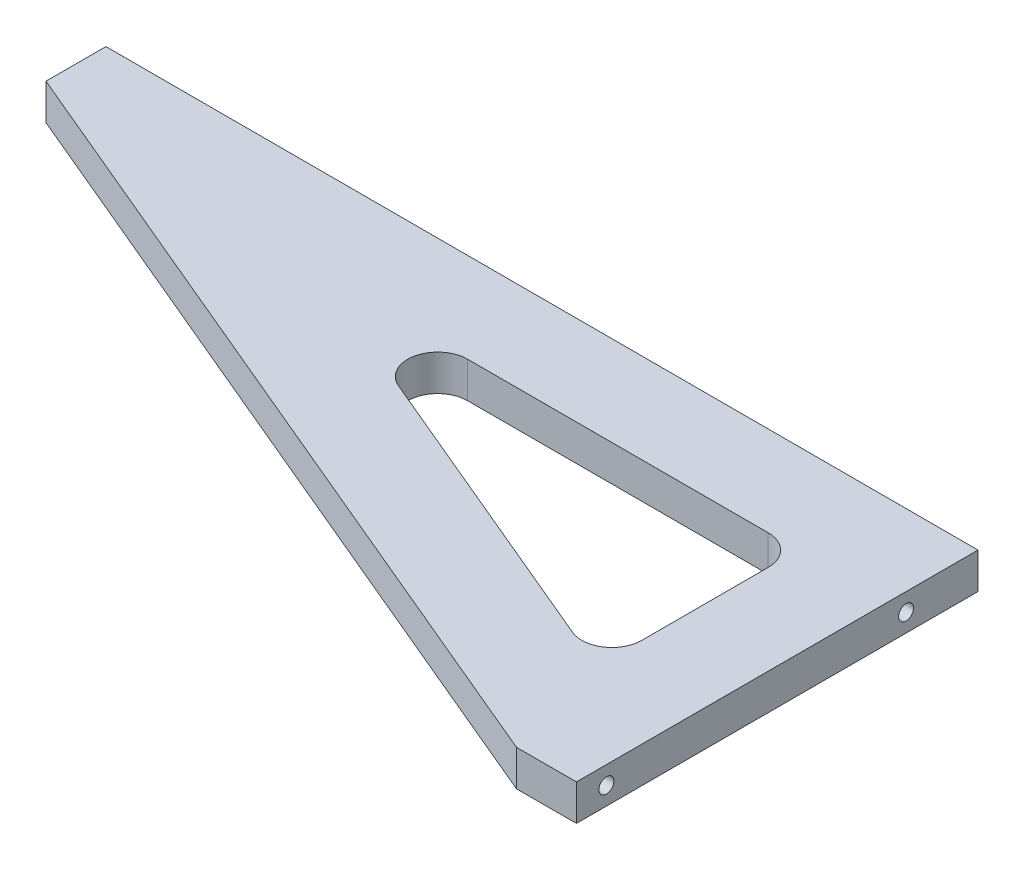
SolidWorks part; units mm, degrees
material "A6061"
ref_plane "前基準面" through (0, 0, 0) normal (0, 0, 1) x (1, 0, 0)
ref_plane "上基準面" through (0, 0, 0) normal (0, 1, 0) x (1, 0, 0)
ref_plane "右基準面" through (0, 0, 0) normal (1, 0, 0) x (0, 0, -1)
sketch "草图1" plane through (0, 0, 0) normal (0, 1, 0) x (1, 0, 0)
  line L1 (-145.5, -67) -> (145.5, -67)
  line L2 (-145.5, -67) -> (-145.5, 67)
  line L3 (-145.5, 67) -> (145.5, 67)
  line L4 (145.5, -67) -> (145.5, 67)
  line L5 (-145.5, -67) -> (145.5, 67) construction
  line L6 (-145.5, 67) -> (145.5, -67) construction
  point P0 (0, 0)
  dimension "D1" = 291
  dimension "D2" = 134
extrude "凸台-拉伸1" add sketch "草图1" along normal mid plane 12
sketch "草图2" plane through (0, 6, 0) normal (0, 1, 0) x (1, 0, 0)
  line L1 (-145.5, -67) -> (125.5, -67)
  line L2 (-145.5, -67) -> (-145.5, 47)
  line L6 (-145.5, 47) -> (125.5, -67)
  line L7 (145.5, -67) -> (145.5, 67) construction
  line L8 (145.5, 67) -> (-145.5, 67) construction
  line L9 (115.5, -15.1916) -> (115.5, 27)
  line L10 (105.5, 37) -> (5.2024, 37)
  line L11 (1.3248, 17.7824) -> (101.6225, -24.4093)
  arc A1 (5.2024, 37) -> (1.3248, 17.7824) centre (5.2024, 27) ccw
  arc A2 (115.5, 27) -> (105.5, 37) centre (105.5, 27) ccw
  arc A3 (115.5, -15.1916) -> (101.6225, -24.4093) centre (105.5, -15.1916) cw
  dimension "D3" = 30
  dimension "D6" = 10
  dimension "D1" = 20
  dimension "D2" = 20
  dimension "D4" = 30
  dimension "D5" = 30
extrude "切除-拉伸1" cut sketch "草图2" against normal through all
hole_wizard "M6 螺纹孔1" positions "草图3" profile "草图4" tap size "M6" standard "GB"
sketch "草图3" plane through (145.5, 0, 0) normal (1, 0, 0) x (0, 0, -1)
  line L0 (-67, 6) -> (-67, -6) construction
  point P0 (-57, 0)
  point P3 (43, 0)
  dimension "D2" = 10
  dimension "D3" = 100
sketch "草图4" plane through (145.5, 0, 57) normal (0, 1, 0) x (0, 0, -1)
  line L0 (0, 0) -> (0, 16.5022)
  line L1 (0, 16.5022) -> (2.5, 15)
  line L2 (2.5, 15) -> (2.5, 0)
  line L5 (2.5, 0) -> (0, 0)
  line L10 (0, 16.5022) -> (-2.5, 15) construction
  line L11 (0, -6.35) -> (0, 107.95) construction
  dimension "螺纹孔钻头直径" = 5
  dimension "螺纹孔钻头深度" = 15
  dimension "导头角度" = 118
cosmetic thread "孔螺蚊线2" parameters "D1"=12, "D2"=6
cosmetic thread "孔螺蚊线3" parameters "D1"=12, "D2"=6
hole_wizard "M6 螺纹孔2" positions "草图5" profile "草图6" tap size "M6" standard "GB"
sketch "草图5" plane through (0, 0, -67) normal (0, 0, -1) x (-1, 0, 0)
  line L0 (145.5, 6) -> (145.5, -6) construction
  point P0 (135.5, 0)
  point P5 (25.5, 0)
  point P6 (-84.5, 0)
  dimension "D2" = 10
  dimension "D3" = 110
  dimension "D1" = 3
sketch "草图6" plane through (-135.5, 0, -67) normal (1, 0, 0) x (0, 1, 0)
  line L0 (0, 0) -> (0, 16.5022)
  line L1 (0, 16.5022) -> (2.5, 15)
  line L2 (2.5, 15) -> (2.5, 0)
  line L5 (2.5, 0) -> (0, 0)
  line L10 (0, 16.5022) -> (-2.5, 15) construction
  line L11 (0, -6.35) -> (0, 107.95) construction
  dimension "螺纹孔钻头直径" = 5
  dimension "螺纹孔钻头深度" = 15
  dimension "导头角度" = 118
cosmetic thread "孔螺蚊线4" parameters "D1"=12, "D2"=6
cosmetic thread "孔螺蚊线5" parameters "D1"=12, "D2"=6
cosmetic thread "孔螺蚊线6" parameters "D1"=12, "D2"=6
